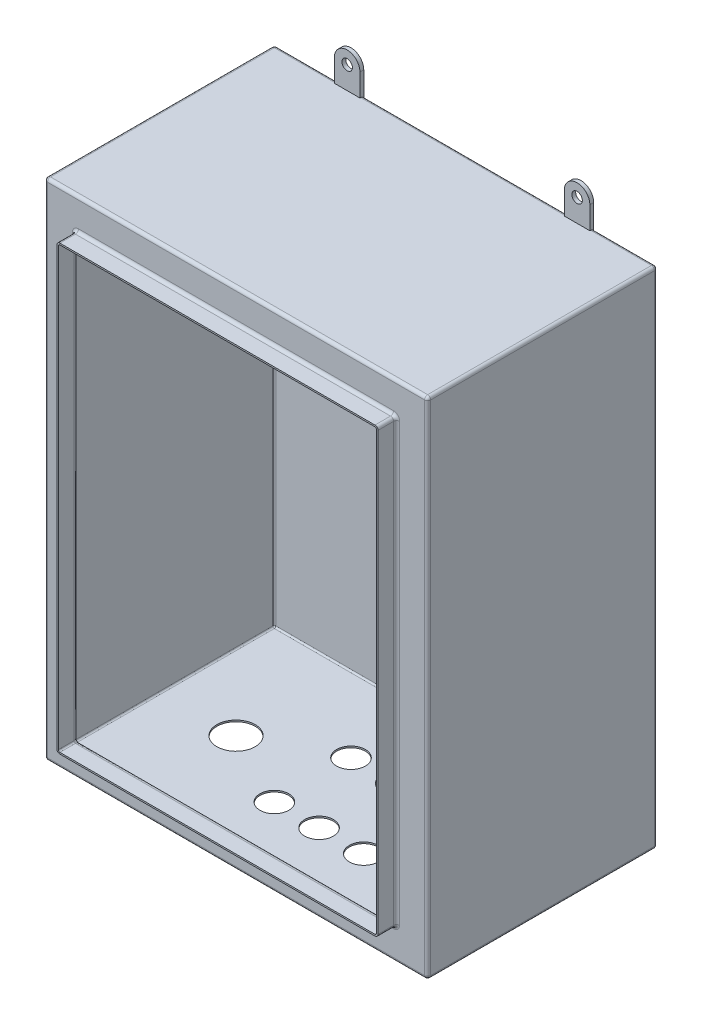
SolidWorks part; units mm, degrees
ref_plane "Front Plane" through (0, 0, 0) normal (0, 0, 1) x (1, 0, 0)
ref_plane "Top Plane" through (0, 0, 0) normal (0, 1, 0) x (1, 0, 0)
ref_plane "Right Plane" through (0, 0, 0) normal (1, 0, 0) x (0, 0, -1)
sketch "Sketch1" plane through (0, 0, 0) normal (0, 1, 0) x (1, 0, 0)
  line L1 (-150, -90) -> (150, -90)
  line L2 (-150, -90) -> (-150, 90)
  line L3 (-150, 90) -> (150, 90)
  line L4 (150, -90) -> (150, 90)
  line L5 (-150, -90) -> (150, 90) construction
  line L6 (-150, 90) -> (150, -90) construction
  point P0 (0, 0)
  dimension "D1" = 300
  dimension "D2" = 180
extrude "Boss-Extrude1" add sketch "Sketch1" along normal blind 395
fillet "Fillet1" radius 2.4 12 edges at (0, 395, 90) (-150, 395, 0) (-150, 0, 0) (0, 0, 90) (0, 395, -90) (-150, 197.5, -90) (0, 0, -90) (150, 197.5, 90) (150, 395, 0) (150, 197.5, -90) (150, 0, 0) (-150, 197.5, 90)
sketch "Sketch2" plane through (0, 0, 90) normal (0, 0, 1) x (1, 0, 0)
  line L0 (147.6, 0) -> (-147.6, 0) construction
  line L1 (-125.74, 370.74) -> (125.74, 370.74)
  line L2 (-125.74, 370.74) -> (-125.74, 24.26)
  line L3 (-125.74, 24.26) -> (125.74, 24.26)
  line L4 (125.74, 370.74) -> (125.74, 24.26)
  line L5 (150, 392.6) -> (150, 2.4) construction
  line L6 (-150, 2.4) -> (-150, 392.6) construction
  dimension "D1" = 24.26
  dimension "D2" = 24.26
  dimension "D3" = 24.26
  dimension "D4" = 346.48
extrude "Boss-Extrude2" add sketch "Sketch2" along normal blind 14.57
fillet "Fillet2" radius 2.4 8 edges at (0, 24.26, 90) (125.74, 197.5, 90) (-125.74, 24.26, 97.285) (125.74, 24.26, 97.285) (125.74, 370.74, 97.285) (-125.74, 370.74, 97.285) (0, 370.74, 90) (-125.74, 197.5, 90)
shell "Shell1" thickness 1.2
sketch "Sketch3" plane through (0, 1.2, 0) normal (0, 1, 0) x (1, 0, 0)
  line L1 (147.6, 90) -> (-147.6, 90) construction
  line L2 (-150, 87.6) -> (-150, -87.6) construction
  circle A0 centre (-90, 0) radius 15
  circle A9 centre (-30, -30) radius 11.25
  circle A10 centre (-30, 30) radius 11.25
  circle A11 centre (5, -30) radius 11.25
  circle A12 centre (5, 30) radius 11.25
  circle A13 centre (40, -30) radius 11.25
  circle A14 centre (40, 30) radius 11.25
  circle A15 centre (75, -30) radius 11.25
  circle A16 centre (75, 30) radius 11.25
  dimension "D1" = 30
  dimension "D2" = 22.5
  dimension "D3" = 22.5
  dimension "D4" = 120
  dimension "D5" = 120
  dimension "D7" = 90
  dimension "D8" = 60
  dimension "D9" = 30
  dimension "D6" = 60
extrude "Cut-Extrude1" cut sketch "Sketch3" against normal through all
sketch "Sketch4" plane through (0, 0, -90) normal (0, 0, -1) x (-1, 0, 0)
  line L0 (-100, 412.6) -> (-100, 393.8)
  line L1 (147.6, 392.6) -> (-147.6, 392.6) construction
  line L3 (-80, 393.8) -> (-80, 412.6)
  line L4 (80, 412.6) -> (80, 393.8)
  line L6 (100, 393.8) -> (100, 412.6)
  line L7 (150, 392.6) -> (150, 2.4) construction
  line L8 (-150, 2.4) -> (-150, 392.6) construction
  line L9 (-100, 1.2) -> (-100, -12.5302)
  line L11 (-80, -12.5302) -> (-80, 1.2)
  line L16 (-100, 393.8) -> (-80, 393.8)
  line L17 (80, 393.8) -> (100, 393.8)
  line L19 (-100, 1.2) -> (-80, 1.2)
  line L20 (80, 1.2) -> (80, -12.5302)
  line L25 (100, -12.5302) -> (100, 1.2)
  line L26 (80, 1.2) -> (100, 1.2)
  circle A0 centre (-90, 412.6) radius 4.1
  arc A1 (-80, 412.6) -> (-100, 412.6) centre (-90, 412.6) ccw
  circle A2 centre (90, 412.6) radius 4.1
  arc A3 (100, 412.6) -> (80, 412.6) centre (90, 412.6) ccw
  arc A7 (-100, -12.5302) -> (-80, -12.5302) centre (-90, -12.5302) ccw
  circle A9 centre (-90, -12.5302) radius 4.1
  arc A10 (80, -12.5302) -> (100, -12.5302) centre (90, -12.5302) ccw
  circle A11 centre (90, -12.5302) radius 4.1
  dimension "D1" = 8.2
  dimension "D2" = 20
  dimension "D4" = 8.2
  dimension "D7" = 8.2
  dimension "D10" = 50
  dimension "D8" = 8.2
  dimension "D3" = 20
  dimension "D5" = 50
  dimension "D6" = 50
  dimension "D9" = 50
extrude "Boss-Extrude3" add sketch "Sketch4" against normal blind 3
